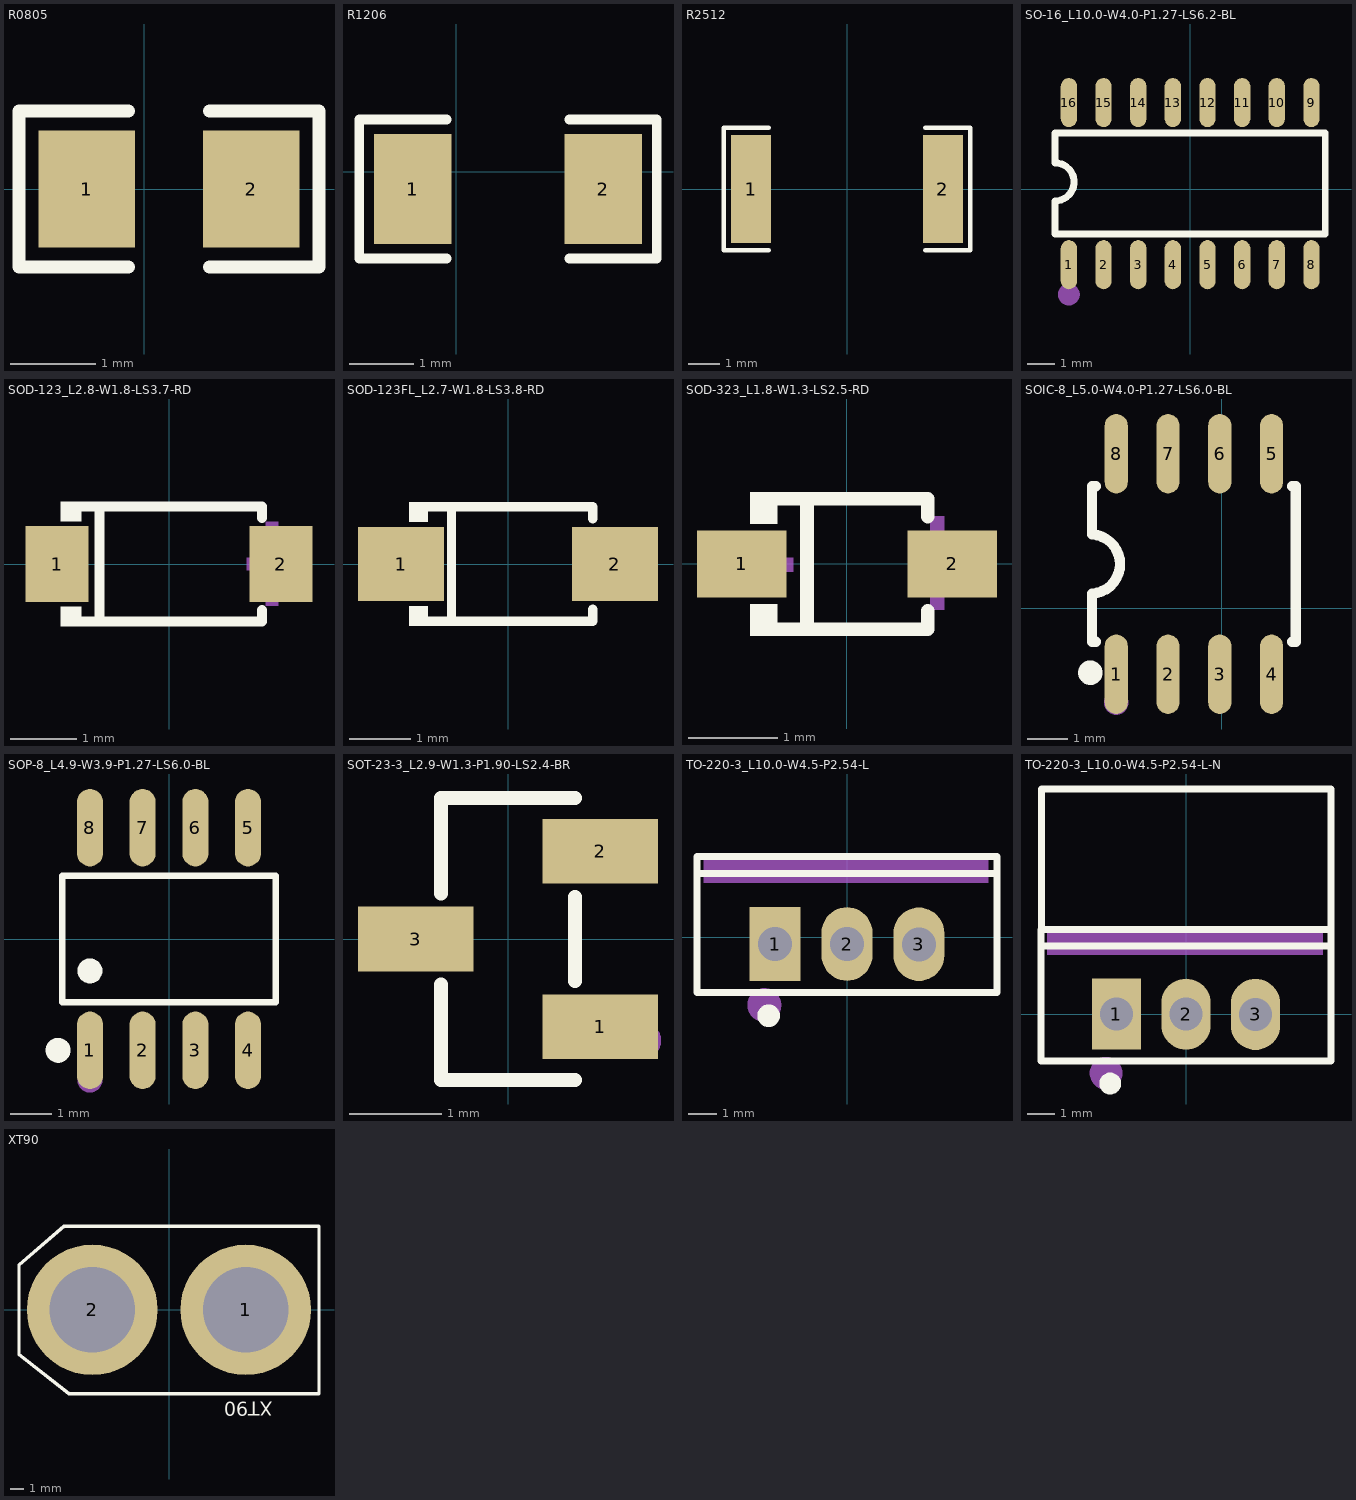
[diagram p0: the footprints below, top view; thin cyan lines are the x and y axes]
# Altium footprint library MISC89356.PcbLib: 29 footprints (part 2 of 2)
Each footprint in its own frame and in the unit in brackets; x right, y up, seen from the top. Pads: shape width x height; smd on the part's side, far side on the other; paste and mask are expansions set on the pad; w line width, h text height; cw(c..) or ccw(c..) is an arc to the next point about the centre after c.

## R0805 [mm]
pads (2):
  rect 1.133x1.377 smd: 1(-0.678,0) 2(1.254,0)
Top Overlay:
  lines w0.152: -0.188,-0.917 -1.473,-0.917 -1.473,0.917 -0.188,0.917 ; 0.764,-0.917 2.049,-0.917 2.049,0.917 0.764,0.917
Top Paste:
  region: 0.738,-0.64 0.738,-0.22 1.183,-0.22 1.183,0.23 0.743,0.23 0.738,0.64 0.788,0.69 1.938,0.69 1.988,0.64 1.988,-0.64 1.938,-0.69 0.788,-0.69
  region: -1.412,-0.64 -1.412,0.64 -1.362,0.69 -0.212,0.69 -0.162,0.64 -0.157,0.23 -0.607,0.23 -0.607,-0.22 -0.167,-0.22 -0.162,-0.64 -0.212,-0.69 -1.362,-0.69

## R1206 [mm]
pads (2):
  rect 1.208x1.701 smd: 1(-0.678,-0.267) 2(2.279,-0.267)
Top Overlay:
  lines w0.152: -0.151,-1.346 -1.511,-1.346 -1.511,0.812 -0.151,0.812 ; 1.751,-1.346 3.111,-1.346 3.111,0.812 1.751,0.812
Top Paste:
  region: -0.075,-1.017 -0.075,-0.656 -0.175,-0.556 -0.385,-0.556 -0.485,-0.456 -0.485,-0.078 -0.385,0.022 -0.175,0.022 -0.075,0.122 -0.075,0.484 -0.175,0.584 -1.182,0.584 -1.282,0.484 -1.282,-1.017 -1.182,-1.117 -0.175,-1.117
  region: 1.675,-1.017 1.675,-0.656 1.775,-0.556 1.986,-0.556 2.086,-0.456 2.086,-0.078 1.986,0.022 1.775,0.022 1.675,0.122 1.675,0.484 1.775,0.584 2.783,0.584 2.883,0.484 2.883,-1.017 2.783,-1.117 1.775,-1.117

## R2512 [mm]
pads (2):
  rect 1.283x3.456 smd: 1(-3.066,0) 2(3.066,0)
Top Overlay:
  lines w0.152: -2.501,-1.957 -3.936,-1.957 -3.936,1.957 -2.501,1.957 ; 2.501,-1.957 3.936,-1.957 3.936,1.957 2.501,1.957
Top Paste:
  region: 2.425,-1.628 2.425,-0.688 2.525,-0.588 2.761,-0.588 2.861,-0.488 2.861,0.488 2.761,0.588 2.525,0.588 2.425,0.688 2.425,1.628 2.525,1.728 3.608,1.728 3.708,1.628 3.708,-1.628 3.608,-1.728 2.525,-1.728
  region: -2.425,-1.628 -2.425,-0.688 -2.525,-0.588 -2.761,-0.588 -2.861,-0.488 -2.861,0.488 -2.761,0.588 -2.525,0.588 -2.425,0.688 -2.425,1.628 -2.525,1.728 -3.608,1.728 -3.708,1.628 -3.708,-1.628 -3.608,-1.728 -2.525,-1.728

## SO-16_L10.0-W4.0-P1.27-LS6.2-BL [mm]
pads (16):
  oval 0.6x1.8 smd: 1(-4.444,-2.776) 2(-3.174,-2.776) 3(-1.904,-2.776) 4(-0.634,-2.776) 5(0.636,-2.776) 6(1.906,-2.776) 7(3.176,-2.776) 8(4.446,-2.776) 9(4.446,3.168) 10(3.176,3.168) 11(1.906,3.168) 12(0.636,3.168) 13(-0.634,3.168) 14(-1.904,3.168) 15(-3.174,3.168) 16(-4.444,3.168)
Top Overlay:
  lines w0.254: -4.952,0.958 cw(c-4.952,0.26) -4.952,-0.439 -4.952,-1.654 -4.949,-1.654 4.952,-1.654 4.952,2.046 -4.949,2.046 -4.949,0.958
Mechanical 15:
  circle w0.4: c-4.444,-3.868 r0.2

## SOD-123_L2.8-W1.8-LS3.7-RD [mm]
pads (2):
  rect 0.95x1.15 smd: 1(-1.693,0) 2(1.693,0)
Top Overlay:
  region: -1.33,-0.942 -1.33,-0.647 -1.635,-0.647 -1.635,-0.942
  region: -1.33,0.942 -1.33,0.647 -1.635,0.647 -1.635,0.942
  lines w0.152: -1.406,-0.866 1.406,-0.866 1.406,-0.698 ; -1.406,0.866 1.406,0.866 1.406,0.698 ; -1.049,-0.866 -1.049,0.866
Mechanical 15:
  region: 1.651,0.635 1.651,-0.629 1.461,-0.629 1.461,0.635
  region: 1.935,0.098 1.935,-0.092 1.177,-0.092 1.177,0.098
  region: -2.03,0.095 -2.03,-0.095 -1.272,-0.095 -1.272,0.095

## SOD-123FL_L2.7-W1.8-LS3.8-RD [mm]
pads (2):
  rect 1.4x1.2 smd: 1(-1.735,0) 2(1.735,0)
Top Overlay:
  region: -1.3,1.002 -1.3,0.682 -1.605,0.682 -1.605,1.002
  region: -1.3,-1.002 -1.3,-0.682 -1.605,-0.682 -1.605,-1.002
  lines w0.152: -1.376,-0.926 1.376,-0.926 1.376,-0.733 ; -1.376,0.926 1.376,0.926 1.376,0.733 ; -0.917,-0.876 -0.917,0.876
Mechanical 15:
  region: -2.032,0.127 -2.032,-0.065 -1.264,-0.065 -1.264,0.127
  region: 2.035,0.096 2.035,-0.096 1.267,-0.096 1.267,0.096
  region: 1.747,-0.384 1.555,-0.384 1.555,0.384 1.747,0.384

## SOD-323_L1.8-W1.3-LS2.5-RD [mm]
pads (2):
  rect 1x0.75 smd: 1(-1.173,0) 2(1.173,0)
Top Overlay:
  region: -0.775,0.802 -0.775,0.45 -1.08,0.45 -1.08,0.802
  region: -0.775,-0.802 -0.775,-0.45 -1.08,-0.45 -1.08,-0.802
  lines w0.152: -0.851,-0.726 0.901,-0.726 0.901,-0.52 ; -0.851,0.726 0.901,0.726 0.901,0.53 ; -0.447,-0.726 -0.447,0.726
Mechanical 15:
  region: -1.225,0.07 -1.225,-0.086 -0.601,-0.086 -0.601,0.07
  region: 1.315,0.09 1.315,-0.066 0.691,-0.066 0.691,0.09
  region: 1.083,0.53 1.083,-0.51 0.927,-0.51 0.927,0.53

## SOIC-8_L5.0-W4.0-P1.27-LS6.0-BL [mm]
pads (8):
  oval 0.568x1.95 smd: 1(-2.59,-1.623) 2(-1.32,-1.623) 3(-0.05,-1.623) 4(1.22,-1.623) 5(1.22,3.787) 6(-0.05,3.787) 7(-1.32,3.787) 8(-2.59,3.787)
Top Overlay:
  circle w0.3: c-3.225,-1.585 r0.15
  lines w0.254: -3.185,1.809 -3.185,2.582 -3.185,2.987 -3.094,2.987 ; -3.18,1.809 cw(c-3.225,1.082) -3.185,0.356 -3.185,-0.418 -3.185,-0.823 -3.094,-0.823 ; 1.723,-0.823 1.815,-0.823 1.815,-0.418 1.815,2.582 1.815,2.987 1.723,2.987
Mechanical 15:
  circle w0.3: c-2.59,-2.318 r0.15

## SOP-8_L4.9-W3.9-P1.27-LS6.0-BL [mm]
pads (8):
  oval 0.63x1.865 smd: 1(-1.905,-2.682) 2(-0.635,-2.682) 3(0.635,-2.682) 4(1.905,-2.682) 5(1.905,2.682) 6(0.635,2.682) 7(-0.635,2.682) 8(-1.905,2.682)
Top Overlay:
  circle w0.3: c-1.905,-0.769 r0.15
  circle w0.3: c-2.672,-2.682 r0.15
  lines w0.152: -2.576,-1.521 -2.576,1.521 2.576,1.521 2.576,-1.521 -2.576,-1.521
Mechanical 15:
  circle w0.3: c-1.905,-3.4 r0.15

## SOT-23-3_L2.9-W1.3-P1.90-LS2.4-BR [mm]
pads (3):
  rect 1.25x0.7 smd: 1(1,-0.95) 2(1,0.95) 3(-1,0)
Top Overlay:
  lines w0.152: -0.726,-0.495 -0.726,-1.526 0.726,-1.526 ; -0.726,0.495 -0.726,1.526 0.726,1.526 ; 0.726,-0.455 0.726,0.455
Mechanical 15:
  circle w0.2: c1.46,-1.1 r0.1

## TO-220-3_L10.0-W4.5-P2.54-L [mm]
pads (3):
  rect 1.8x2.6 hole 1.2: 1(-2.54,-0.241)
  oval 1.8x2.6 hole 1.2: 2(0,-0.241) 3(2.54,-0.251)
Top Overlay:
  lines w0.254: -5.3,2.249 5.3,2.249 ; -5.301,-1.95 5.301,-1.95 5.301,2.849 -5.301,2.849 -5.301,2.843 -5.301,-1.95
  lines w0.4: -2.77,-2.576 ccw(c-2.769,-2.776) -2.767,-2.576
Mechanical 15:
  circle w0.6: c-2.921,-2.4 r0.3
  region: -5.06,2.765 -5.06,1.925 4.99,1.925 4.99,2.765

## TO-220-3_L10.0-W4.5-P2.54-L-N [mm]
pads (3):
  rect 1.8x2.6 hole 1.2: 1(-2.54,0.005)
  oval 1.8x2.6 hole 1.2: 2(0,0.005) 3(2.54,-0.005)
Top Overlay:
  lines w0.254: -5.3,2.495 5.3,2.495 ; -5.301,3.094 -5.301,3.089 -5.301,-1.704 5.301,-1.704 5.301,3.094 ; -5.301,3.094 5.301,3.094 ; -5.301,3.094 -5.28,3.094 -5.28,7.64 -5.28,8.23 5.301,8.23 5.301,3.094
  lines w0.4: -2.77,-2.33 ccw(c-2.769,-2.53) -2.767,-2.33
Mechanical 15:
  circle w0.6: c-2.921,-2.154 r0.3
  region: -5.06,3.01 -5.06,2.17 4.99,2.17 4.99,3.01

## XT90 [mm]
pads (2):
  round 9.5 hole 6.2: 1(5.588,0) 2(-5.588,0)
Top Overlay:
  lines w0.254: -10.922,-3.263 -10.922,3.263 -7.62,6.096 10.922,6.096 10.922,-6.096 -7.295,-6.096 -10.922,-3.263
  text "XT90" at 7.556,-6.708 h1.02